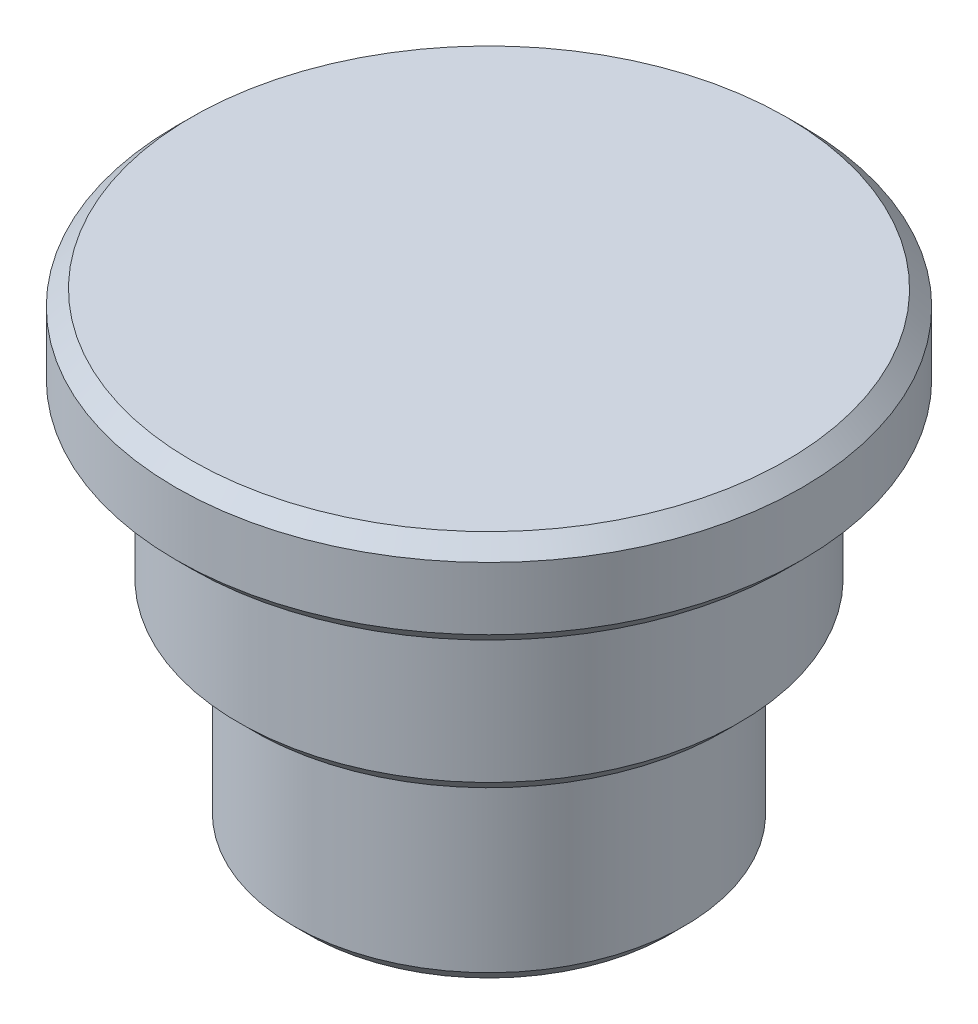
from build123d import *

# Parameters (mm, degrees)
CHAMFER1_SIZE = 0.5


with BuildPart() as part:
    # Sketch1 → Revolve1 (revolve)
    with BuildSketch(Plane.XY, mode=Mode.PRIVATE) as revolve1_sk:
        Polygon((88.713048819, -48.25), (88.713048819, -41.75), (90.463048819, -41.75), (90.463048819, -36.25), (92.463048819, -36.25), (92.463048819, -33.25), (82.463048819, -33.25), (82.463048819, -48.25), align=None)
    revolve(revolve1_sk.sketch.rotate(Axis((82.463048819, -48.25, 0), (0, 1, 0)), 90), axis=Axis((82.463048819, -48.25, 0), (0, 1, 0)))

    # Chamfer1
    chamfer1_edges = [part.edges().sort_by_distance(p)[0] for p in [
        (82.463048819, -33.25, 10),
        (82.463048819, -36.25, 10),
        (82.463048819, -41.75, 8),
        (82.463048819, -48.25, 6.25),
    ]]
    chamfer(chamfer1_edges, length=CHAMFER1_SIZE)


solid = part.part
